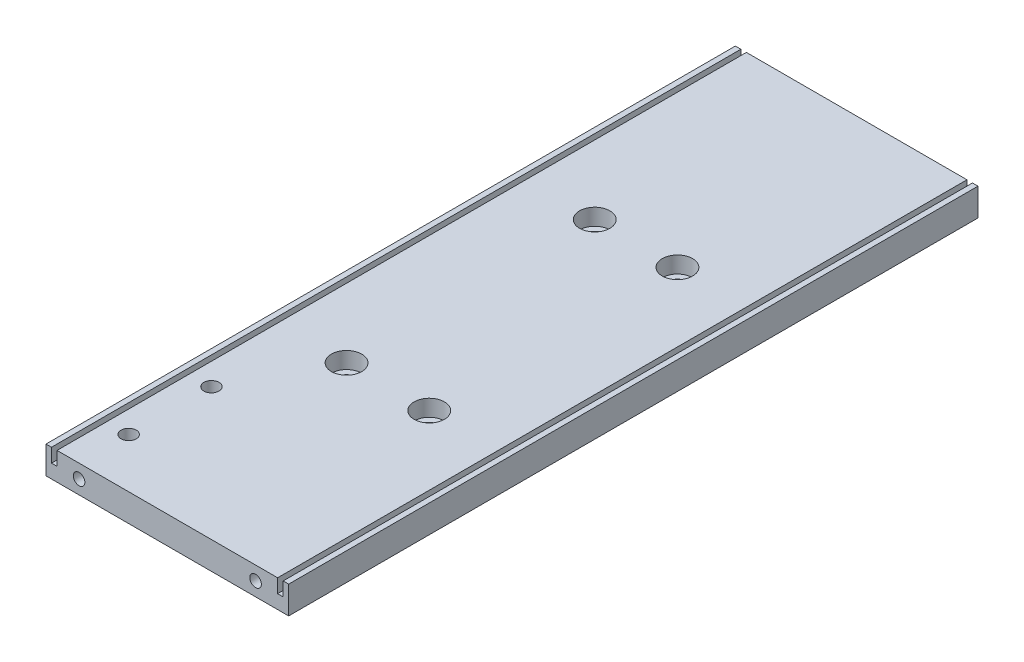
SolidWorks part; units mm, degrees
material "6061 合金"
ref_plane "前视基准面" through (0, 0, 0) normal (0, 0, 1) x (1, 0, 0)
ref_plane "上视基准面" through (0, 0, 0) normal (0, 1, 0) x (1, 0, 0)
ref_plane "右视基准面" through (0, 0, 0) normal (1, 0, 0) x (0, 0, -1)
sketch "草图1" plane through (0, 0, 0) normal (0, 0, 1) x (1, 0, 0)
  line L1 (-44, 5) -> (44, 5)
  line L2 (-44, 5) -> (-44, -5)
  line L3 (-44, -5) -> (44, -5)
  line L4 (44, 5) -> (44, -5)
  line L5 (-44, 5) -> (44, -5) construction
  line L6 (-44, -5) -> (44, 5) construction
  point P0 (0, 0)
  dimension "D1" = 88
  dimension "D2" = 10
extrude "凸台-拉伸1" add sketch "草图1" along normal blind 250
sketch "草图2" plane through (0, 0, 250) normal (0, 0, 1) x (1, 0, 0)
  line L0 (0, 20.0767) -> (0, -21.4003) construction
  line L1 (-40, 5) -> (-40, 0)
  line L2 (40, 5) -> (40, 0)
  line L3 (-42, 5) -> (-42, 0)
  line L4 (42, 5) -> (42, 0)
  line L5 (-42, 5) -> (-40, 5)
  line L6 (-40, 0) -> (-42, 0)
  line L7 (44, 0) -> (-44, 0)
  line L8 (42, 0) -> (40, 0)
  line L9 (-40, 20.0767) -> (-40, -21.4003) construction
  line L10 (-42, 20.0767) -> (-42, -21.4003) construction
  line L11 (44, 5) -> (-44, 5) construction
  line L12 (40, 5) -> (42, 5)
  line L14 (40, 20.0767) -> (40, -21.4003) construction
  line L15 (42, 20.0767) -> (42, -21.4003) construction
  dimension "D1" = 40
  dimension "D2" = 40
  dimension "D3" = 2
  dimension "D4" = 2
  dimension "D5" = 5
extrude "切除-拉伸1" cut sketch "草图2" against normal through all
sketch "草图3" plane through (0, 0, 250) normal (0, 0, 1) x (1, 0, 0)
  line L0 (0, 21.4461) -> (0, -26.1482) construction
  line L1 (-32, 21.4461) -> (-32, -26.1482) construction
  line L2 (32, 21.4461) -> (32, -26.1482) construction
  line L3 (-52.2328, 0) -> (56.4544, 0) construction
  dimension "D1" = 32
  dimension "D2" = 32
hole_wizard "M5 螺纹孔1" positions "3D草图1" profile "草图4" tap size "M5" standard "GB"
sketch3d "3D草图1"
  line L0 (-32, 21.4461, 250) -> (-32, -26.1482, 250) construction
  line L1 (-52.2328, 0, 250) -> (56.4544, 0, 250) construction
  line L2 (32, 21.4461, 250) -> (32, -26.1482, 250) construction
  point P0 (-32, 0, 250)
  point P6 (32, 0, 250)
sketch "草图4" plane through (-32, 0, 250) normal (1, 0, 0) x (0, -1, 0)
  line L0 (0, 0) -> (0, 11.2618)
  line L1 (0, 11.2618) -> (2.1, 10)
  line L2 (2.1, 10) -> (2.1, 0)
  line L5 (2.1, 0) -> (0, 0)
  line L10 (0, 11.2618) -> (-2.1, 10) construction
  line L11 (0, -6.35) -> (0, 107.95) construction
  dimension "螺纹孔钻头直径" = 4.2
  dimension "螺纹孔钻头深度" = 10
  dimension "导头角度" = 118
cosmetic thread "孔螺蚊线1" parameters "D1"=10, "D2"=5
cosmetic thread "孔螺蚊线2" parameters "D1"=10, "D2"=5
sketch "草图5" plane through (0, 0, 0) normal (0, 0, -1) x (-1, 0, 0)
  line L0 (-62.6004, 0) -> (59.6929, 0) construction
  line L1 (-32, 12.5208) -> (-32, -11.1179) construction
  line L2 (32, 10.3922) -> (32, -15.5992) construction
hole_wizard "M5 螺纹孔2" positions "3D草图2" profile "草图6" tap size "M5" standard "GB"
sketch3d "3D草图2"
  line L0 (62.6004, 0, 0) -> (-59.6929, 0, 0) construction
  line L1 (32, 12.5208, 0) -> (32, -11.1179, 0) construction
  line L2 (-32, 10.3922, 0) -> (-32, -15.5992, 0) construction
  point P0 (32, 0, 0)
  point P6 (-32, 0, 0)
sketch "草图6" plane through (32, 0, 0) normal (1, 0, 0) x (0, 1, 0)
  line L0 (0, 0) -> (0, 11.2618)
  line L1 (0, 11.2618) -> (2.1, 10)
  line L2 (2.1, 10) -> (2.1, 0)
  line L5 (2.1, 0) -> (0, 0)
  line L10 (0, 11.2618) -> (-2.1, 10) construction
  line L11 (0, -6.35) -> (0, 107.95) construction
  dimension "螺纹孔钻头直径" = 4.2
  dimension "螺纹孔钻头深度" = 10
  dimension "导头角度" = 118
cosmetic thread "孔螺蚊线3" parameters "D1"=10, "D2"=5
cosmetic thread "孔螺蚊线4" parameters "D1"=10, "D2"=5
sketch "草图7" plane through (0, 5, 0) normal (0, 1, 0) x (1, 0, 0)
  line L0 (-103.0297, -125) -> (118.4606, -125) construction
  line L1 (-103.0297, -170) -> (118.4606, -170) construction
  line L2 (-103.0297, -80) -> (118.4606, -80) construction
  line L3 (0, 26.3247) -> (0, -284.9975) construction
  circle A0 centre (-15, -80) radius 3.25
  circle A1 centre (15, -80) radius 3.25
  circle A2 centre (15, -170) radius 3.25
  circle A3 centre (-15, -170) radius 3.25
  dimension "D3" = 30
  dimension "D4" = 6.5
  dimension "D1" = 45
  dimension "D2" = 45
extrude "切除-拉伸2" cut sketch "草图7" against normal through all
sketch "草图8" plane through (0, 5, 0) normal (0, 1, 0) x (1, 0, 0)
  circle A0 centre (-15, -80) radius 5.5
  circle A1 centre (15, -80) radius 5.5
  circle A2 centre (-15, -170) radius 5.5
  circle A3 centre (15, -170) radius 5.5
  dimension "D1" = 11
  dimension "D2" = 11
  dimension "D3" = 11
  dimension "D4" = 11
extrude "切除-拉伸3" cut sketch "草图8" against normal blind 6
sketch "草图9" plane through (0, -5, 0) normal (0, -1, 0) x (1, 0, 0)
  line L0 (0, 235.118) -> (0, -15.4529) construction
  line L1 (32, 235.118) -> (32, 232) construction
  line L5 (-32, 235.118) -> (-32, -15.4529) construction
  line L6 (-13.1891, 202) -> (-60.5524, 202) construction
  line L7 (-22.6097, 232) -> (-58.1909, 232) construction
  line L8 (32, 202) -> (32, -15.4529) construction
  line L10 (32, 229.25) -> (32, 204.75) construction
  line L11 (32, 235.118) -> (32, -15.4529) construction
  circle A2 centre (-32, 232) radius 2.75
  circle A3 centre (-32, 202) radius 2.75
  point P8 (15, 202)
  point P9 (53.8217, 202)
  point P10 (15, 232)
  point P11 (53.8217, 232)
  dimension "D7" = 5.5
  dimension "D8" = 5.5
  dimension "D6" = 32
extrude "切除-拉伸4" cut sketch "草图9" against normal through all
sketch "草图10" plane through (0, -5, 0) normal (0, -1, 0) x (1, 0, 0)
  circle A0 centre (-32, 232) radius 4.5
  circle A1 centre (-32, 202) radius 4.5
  dimension "D1" = 9
  dimension "D2" = 9
extrude "切除-拉伸5" cut sketch "草图10" against normal blind 5
